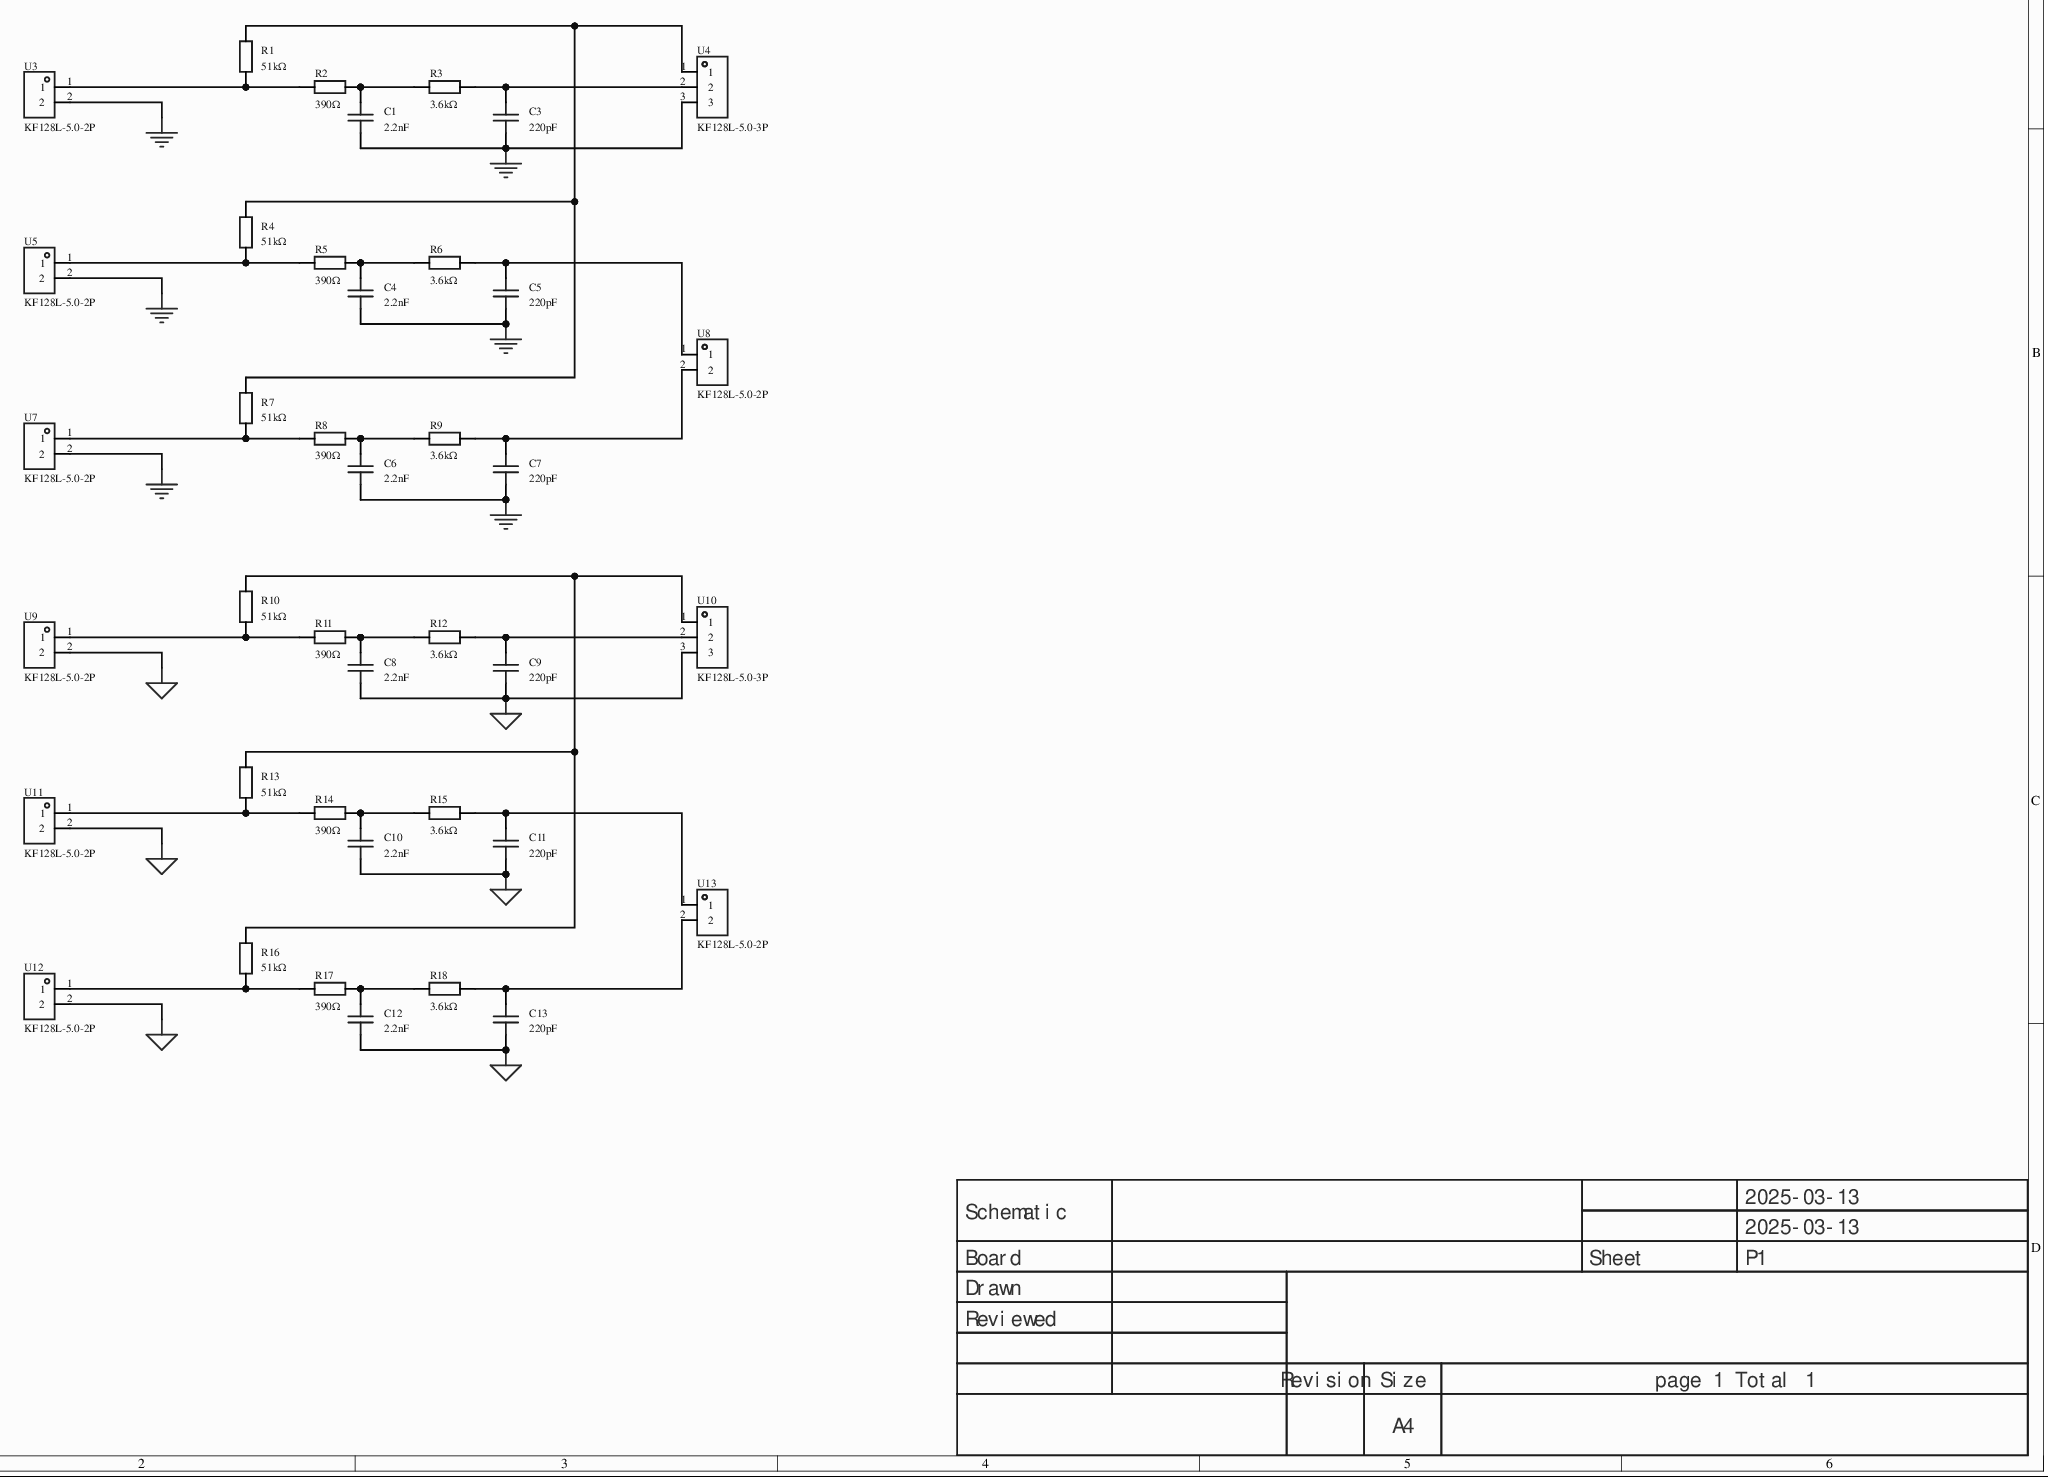
[diagram p0: MISC52125-3.schdoc]
# Altium project MISC52125-2.PrjPcb
1 sheet, 40 parts. Net scope: global (net labels, ports and power ports of the same name join across sheets).
Board file: MISC52125.pcbdoc

## Sheet MISC52125-3.schdoc
size 420 x 297 mm; Version: V1.0; @Project Name: MISC52125; @Page Count: 1; @Update Date: 2025-03-13; @Create Date: 2025-03-13; @Schematic Name: MISC52125; @Page No: 1; @Create Time: 16:58:12; @Update Time: 16:58:12; @Board Name: MISC52125

### Parts
C1  2.2nF  [CAP-TH_L8.0-W5.0-P7.50-D1.0]
C3  220pF  [CAP-TH_L7.2-W4.5-P5.00-D0.5]
C4  2.2nF  [CAP-TH_L8.0-W5.0-P7.50-D1.0]
C5  220pF  [CAP-TH_L7.2-W4.5-P5.00-D0.5]
C6  2.2nF  [CAP-TH_L8.0-W5.0-P7.50-D1.0]
C7  220pF  [CAP-TH_L7.2-W4.5-P5.00-D0.5]
C8  2.2nF  [CAP-TH_L8.0-W5.0-P7.50-D1.0]
C9  220pF  [CAP-TH_L7.2-W4.5-P5.00-D0.5]
C10  2.2nF  [CAP-TH_L8.0-W5.0-P7.50-D1.0]
C11  220pF  [CAP-TH_L7.2-W4.5-P5.00-D0.5]
C12  2.2nF  [CAP-TH_L8.0-W5.0-P7.50-D1.0]
C13  220pF  [CAP-TH_L7.2-W4.5-P5.00-D0.5]
R1  51kΩ  [Res_1/4W]
R2  390Ω  [Res_1/4W]
R3  3.6kΩ  [Res_1/4W]
R4  51kΩ  [Res_1/4W]
R5  390Ω  [Res_1/4W]
R6  3.6kΩ  [Res_1/4W]
R7  51kΩ  [Res_1/4W]
R8  390Ω  [Res_1/4W]
R9  3.6kΩ  [Res_1/4W]
R10  51kΩ  [Res_1/4W]
R11  390Ω  [Res_1/4W]
R12  3.6kΩ  [Res_1/4W]
R13  51kΩ  [Res_1/4W]
R14  390Ω  [Res_1/4W]
R15  3.6kΩ  [Res_1/4W]
R16  51kΩ  [Res_1/4W]
R17  390Ω  [Res_1/4W]
R18  3.6kΩ  [Res_1/4W]
U3  KF128L-5.0-2P  [CONN-TH_P5.00_KF128L-5.0-2P]
U4  KF128L-5.0-3P  [CONN-TH_3P-P5.00_KF128L-5.0-3P]
U5  KF128L-5.0-2P  [CONN-TH_P5.00_KF128L-5.0-2P]
U7  KF128L-5.0-2P  [CONN-TH_P5.00_KF128L-5.0-2P]
U8  KF128L-5.0-2P  [CONN-TH_P5.00_KF128L-5.0-2P]
U9  KF128L-5.0-2P  [CONN-TH_P5.00_KF128L-5.0-2P]
U10  KF128L-5.0-3P  [CONN-TH_3P-P5.00_KF128L-5.0-3P]
U11  KF128L-5.0-2P  [CONN-TH_P5.00_KF128L-5.0-2P]
U12  KF128L-5.0-2P  [CONN-TH_P5.00_KF128L-5.0-2P]
U13  KF128L-5.0-2P  [CONN-TH_P5.00_KF128L-5.0-2P]

### Nets
AGND: C8.1 C9.1 C10.1 C11.1 C12.1 C13.1 U9.2 U10.3 U11.2 U12.2
GND: C1.1 C3.1 C4.1 C5.1 C6.1 C7.1 U3.2 U4.3 U5.2 U7.2
NetC1_2: C1.2 R2.1 R3.2
NetC3_2: C3.2 R3.1 U4.2
NetC4_2: C4.2 R5.1 R6.2
NetC5_2: C5.2 R6.1 U8.1
NetC6_2: C6.2 R8.1 R9.2
NetC7_2: C7.2 R9.1 U8.2
NetC8_2: C8.2 R11.1 R12.2
NetC9_2: C9.2 R12.1 U10.2
NetC10_2: C10.2 R14.1 R15.2
NetC11_2: C11.2 R15.1 U13.1
NetC12_2: C12.2 R17.1 R18.2
NetC13_2: C13.2 R18.1 U13.2
NetR1_1: R1.1 R2.2 U3.1
NetR1_2: R1.2 R4.2 R7.2 U4.1
NetR4_1: R4.1 R5.2 U5.1
NetR7_1: R7.1 R8.2 U7.1
NetR10_1: R10.1 R11.2 U9.1
NetR10_2: R10.2 R13.2 R16.2 U10.1
NetR13_1: R13.1 R14.2 U11.1
NetR16_1: R16.1 R17.2 U12.1

### Notes on the sheet
- 2025-03-13
- Schematic
- Board
- Sheet
- P1
- Drawn
- Reviewed
- Revision
- Size
- A4
- page 1 Total 1

### Library data of the parts
C1 C4 C6 C8 C10 C12 = DE2E3KY222MA3BU02F: component DE2E3KY222MA3BU02F capacitance:2.2nF;tolerance:±20%;voltage(AC):300V;class:X1,Y2;; Manufacturer: muRata(村田); AddInBom: yes; ModelId: 891483702e3d4cd188688a4834031f3d; ModelName: CAP-TH_L8.0-W5.0-H11.0-P7.0; ModelTransform: 314.96,196.85,0,0,0,0,0,0,-137.795; Tolerance: ±20%; Voltage(AC): 300V; Subclass: X1,Y2; Symbol: DE2E3KY222MA3BU02F; Device: DE2E3KY222MA3BU02F; LCSC Part Name: 等级:X1,Y2 2.2nF ±20% 300V; SupplierPart: C237450; ManufacturerPart: DE2E3KY222MA3BU02F; Supplier Footprint: 插件,P=7.5mm; JLCPCB Part Class: parameter JLCPCB Part Class  Extended library; Datasheet: https://atta.szlcsc.com/upload/public/pdf/source/20191022/C440140_7AB5F4B3B56EC7AEB2A782F4DBA79A52.pdf; Supplier: LCSC; ConvertToPcb: yes; FootprintName: CAP-TH_L8.0-W5.0-P7.50-D1.0; Value: 2.2nF; Operating Temperature: -40℃~+125℃
C3 C5 C7 C9 C11 C13 = KP1830122633: component KP1830122633 compo capacitance:220pF;tolerance:±2.5%;rated voltage:630V; 250V;operating temperature:-55℃~+100℃;; Manufacturer: VISHAY(威世); AddInBom: yes; ModelId: 5b8f94d09378482e8a7d7c1f412bd9bb; ModelTransform: 283.464,177.165,0,0,0,0,0,0,-196.85; Tolerance: ±2.5%; Symbol: KP1830122633; Device: KP1830122633; LCSC Part Name: 220pF ±2.5% 630V 250V; SupplierPart: C3794724; ManufacturerPart: KP1830122633; Supplier Footprint: 插件,P=5mm; JLCPCB Part Class: parameter JLCPCB Part Class  Extended library; Datasheet: https://atta.szlcsc.com/upload/public/pdf/source/20231212/3165E97C240197E63CE9BCA704937F9C.pdf; Supplier: LCSC; ConvertToPcb: yes; FootprintName: CAP-TH_L7.2-W4.5-P5.00-D0.5; ModelName: CAP-TH_L7.2-W4.5-P5.00-D0.5; Value: 220pF; Voltage Rated: 630V; 250V; Operating Temperature: -55℃~+100℃
R1-R18 = Res_AXIAL-1/4W: AddInBom: yes; SymbolName: parameter SymbolName text    Resistor; ModelId: 463263665006444ab7a47bd11b0cf956; ModelName: RES-TH_BD2.4-L6.3-P10.30-D0.6; ModelTransform: 427.165,94.32816,0,0,0,0,0,0,-196.85; Device: Res_AXIAL-1/4W; Supplier Footprint: 轴向引线; ConvertToPcb: yes; FootprintName: Res_1/4W
  R1 R4 R7 R10 R13 R16: Value: 51kΩ
  R2 R5 R8 R11 R14 R17: Value: 390Ω
  R3 R6 R9 R12 R15 R18: Value: 3.6kΩ
U3 U5 U7-U9 U11-U13 = KF128L-5.0-2P: 可拼接 铜 环保; Manufacturer: KEFA(科发); AddInBom: yes; ModelId: 47f8164fd4864a8399fbdd6534ee28ae; ModelTransform: 405.511,393.7,0,0,0,0,5.906,-3.937,-169.291; Symbol: KF128L-5.0-2P; Device: KF128L-5.0-2P; LCSC Part Name: 间距P=5.0mm 2Pin位 直插 直针 可拼接 铜 环保; SupplierPart: C474938; ManufacturerPart: KF128L-5.0-2P; Supplier Footprint: P=5mm; JLCPCB Part Class: parameter JLCPCB Part Class  Extended library; Datasheet: https://atta.szlcsc.com/upload/public/pdf/source/20230317/752C0AC053DC32F5BE41F95D5E9BCBBC.pdf; Supplier: LCSC; ConvertToPcb: yes; FootprintName: CONN-TH_P5.00_KF128L-5.0-2P; ModelName: CONN-TH_P5.00_KF128L-5.0-2P
U4 U10 = KF128L-5.0-3P: 可拼接 铜 环保; Manufacturer: KEFA(科发); AddInBom: yes; ModelId: cc3e985db2e2444581f9de0f33be2442; ModelTransform: 602.361,393.7,0,0,0,0,5.906,-3.937,-169.291; Symbol: KF128L-5.0-3P; Device: KF128L-5.0-3P; LCSC Part Name: 间距P=5.0mm 3Pin位 直插 直针 可拼接 铜 环保; SupplierPart: C474939; ManufacturerPart: KF128L-5.0-3P; Supplier Footprint: P=5mm; JLCPCB Part Class: parameter JLCPCB Part Class  Extended library; Datasheet: https://atta.szlcsc.com/upload/public/pdf/source/20230317/752C0AC053DC32F5BE41F95D5E9BCBBC.pdf; Supplier: LCSC; ConvertToPcb: yes; FootprintName: CONN-TH_3P-P5.00_KF128L-5.0-3P; ModelName: CONN-TH_3P-P5.00_KF128L-5.0-3P